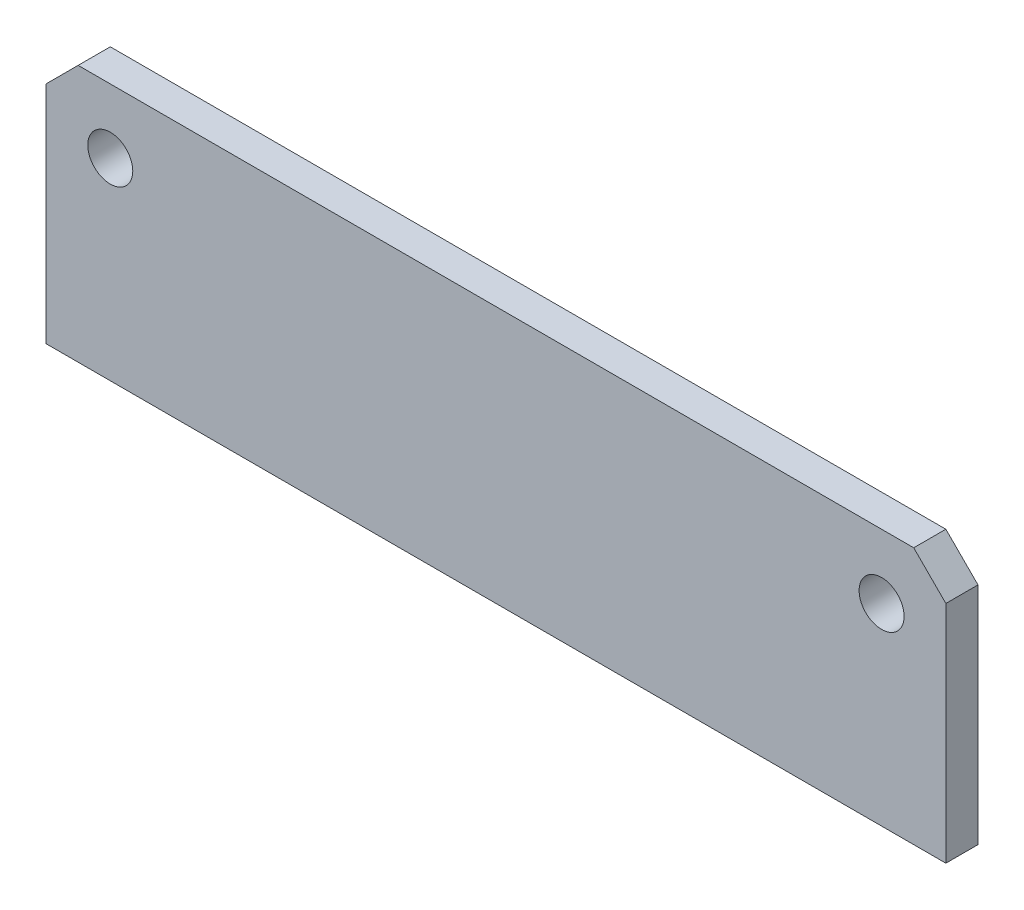
SolidWorks part; units mm, degrees
material "1023 碳钢板 (SS)"
ref_plane "前视基准面" through (0, 0, 0) normal (0, 0, 1) x (1, 0, 0)
ref_plane "上视基准面" through (0, 0, 0) normal (0, 1, 0) x (1, 0, 0)
ref_plane "右视基准面" through (0, 0, 0) normal (1, 0, 0) x (0, 0, -1)
sketch "草图1" plane through (0, 0, 0) normal (0, 0, 1) x (1, 0, 0)
  line L1 (70, 20) -> (-70, 20)
  line L2 (70, 20) -> (70, -20)
  line L3 (70, -20) -> (-70, -20)
  line L4 (-70, 20) -> (-70, -20)
  line L5 (70, 20) -> (-70, -20) construction
  line L6 (70, -20) -> (-70, 20) construction
  point P0 (0, 0)
  dimension "D1" = 140
  dimension "D2" = 40
extrude "凸台-拉伸1" add sketch "草图1" along normal blind 5
sketch "草图2" plane through (0, 0, 5) normal (0, 0, 1) x (1, 0, 0)
  line L0 (70, 20) -> (-70, 20) construction
  line L1 (70, -20) -> (70, 20) construction
  circle A0 centre (-60, 10) radius 3.5
  circle A1 centre (60, 10) radius 3.5
  point P8 (0, 0)
  dimension "D3" = 7
  dimension "D4" = 7
  dimension "D5" = 10
  dimension "D1" = 120
  dimension "D2" = 10
extrude "切除-拉伸1" cut sketch "草图2" against normal blind 5
chamfer "倒角1" distance 5 angle 45 2 edges at (70, 20, 2.5) (-70, 20, 2.5)
